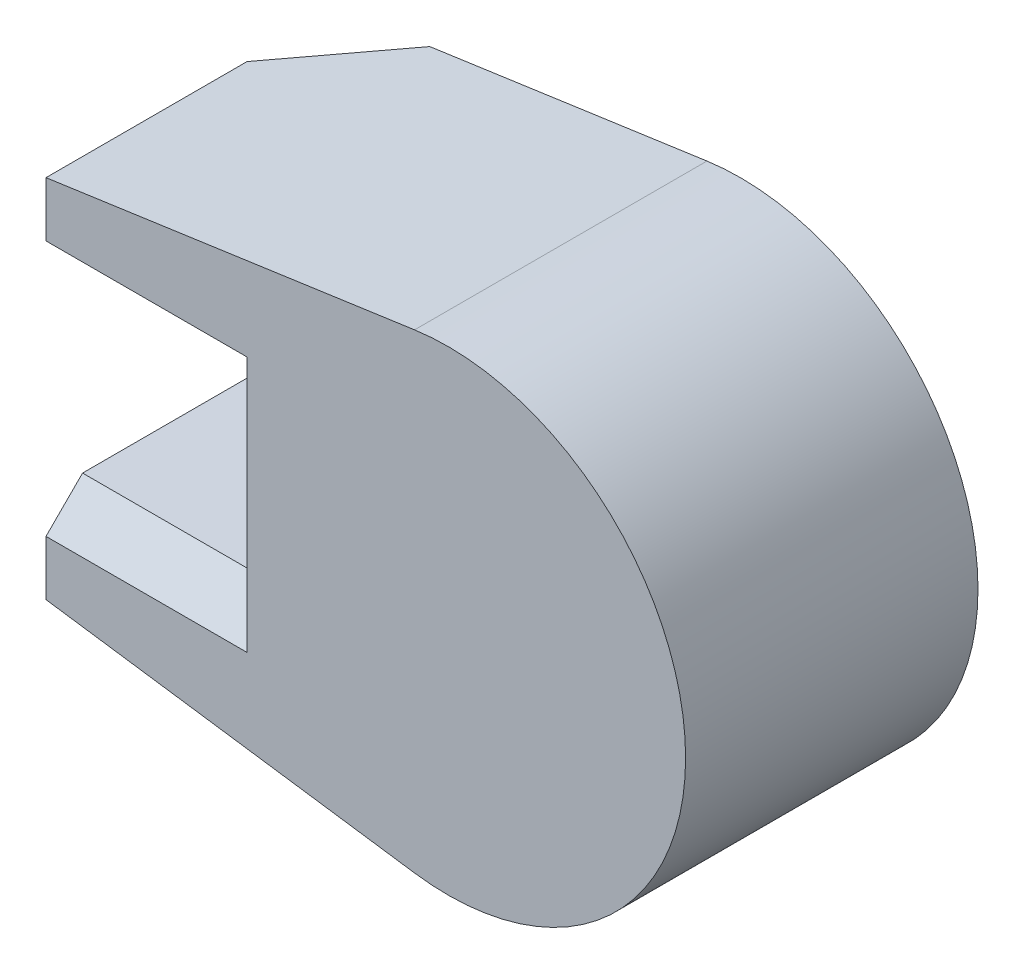
from build123d import *

# Parameters (mm, degrees)
EXTRUDE_1_DEPTH = 40
CHAMFER_1_SIZE  = 25
CHAMFER_2_SIZE  = 10
CHAMFER_3_SIZE  = 10


with BuildPart() as part:
    # 草图1 → 凸台-拉伸1 (new, symmetric)
    with BuildSketch(Plane.XY):
        with BuildLine():
            Line((-110, 50), (-110, 25))
            Line((-110, 25), (-65, 25))
            Line((-65, 25), (-65, -25))
            Line((-65, -25), (-110, -25))
            Line((-110, -25), (-110, -50))
            Line((-110, -50), (-9.158378918, -64.35156638))
            ThreePointArc((-9.158378918, -64.35156638), (65, 0), (-9.158378918, 64.35156638))
            Line((-9.158378918, 64.35156638), (-110, 50))
        make_face()
    extrude(amount=EXTRUDE_1_DEPTH, both=True)

    # 倒角1
    chamfer_1_edges = [part.edges().sort_by_distance(p)[0] for p in [
        (-110, 37.5, -40),
        (-110, -37.5, -40),
    ]]
    chamfer(chamfer_1_edges, length=CHAMFER_1_SIZE)

    # 倒角2
    chamfer_2_edges = [part.edges().sort_by_distance(p)[0] for p in [
        (-87.5, 25, 40),
        (-65, 0, 40),
        (-87.5, -25, 40),
    ]]
    chamfer(chamfer_2_edges, length=CHAMFER_2_SIZE)

    # 倒角3
    chamfer_3_edges = [part.edges().sort_by_distance(p)[0] for p in [
        (-75, 25, -40),
        (-75, -25, -40),
        (-65, 0, -40),
    ]]
    chamfer(chamfer_3_edges, length=CHAMFER_3_SIZE)


solid = part.part
